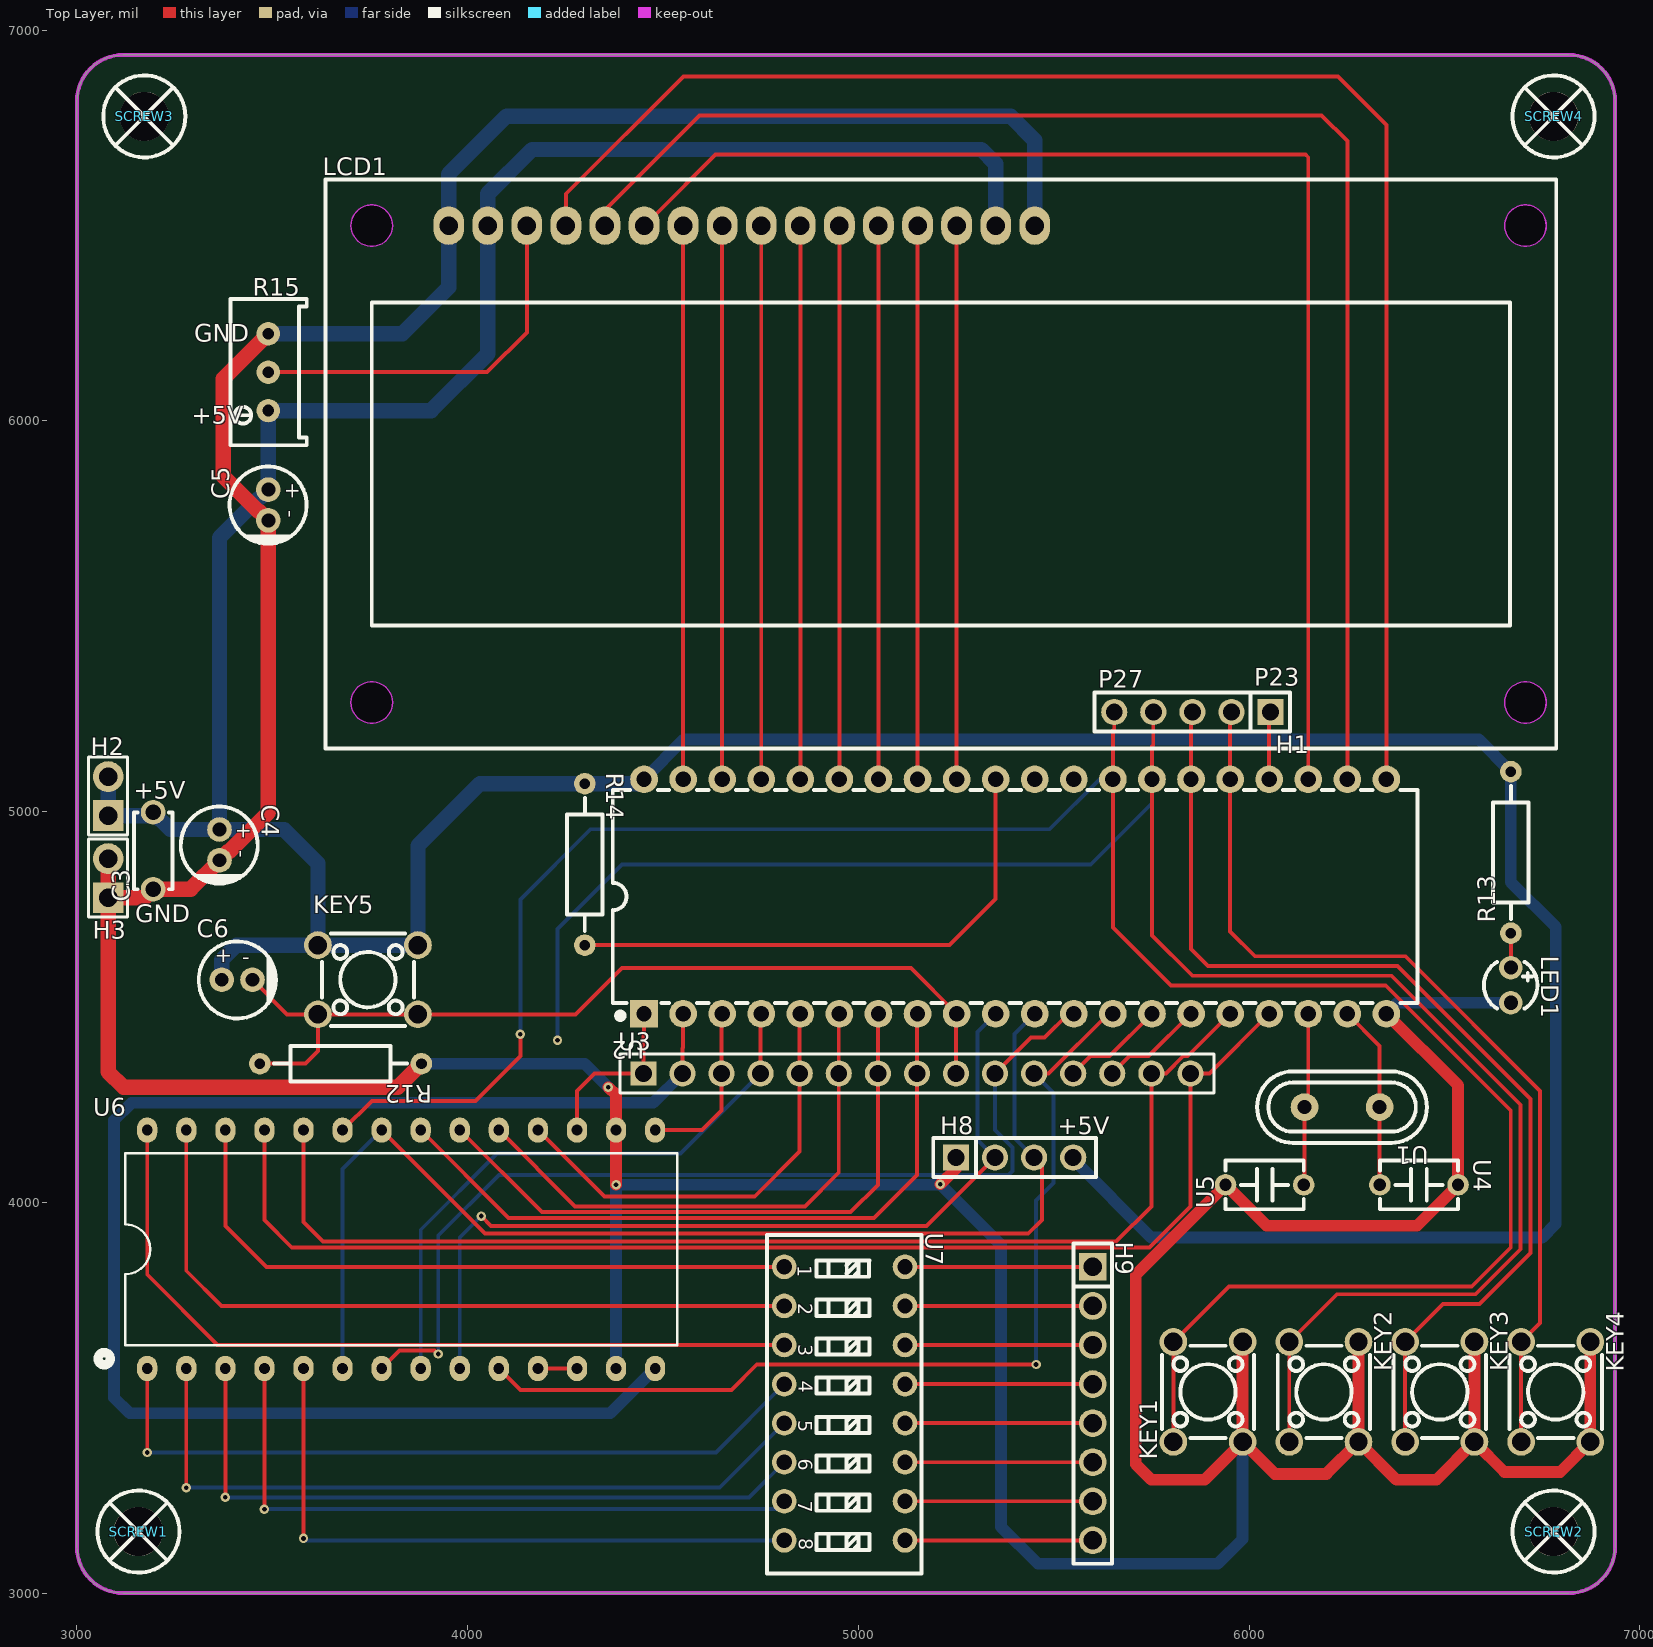
[diagram p0: Top Layer view]
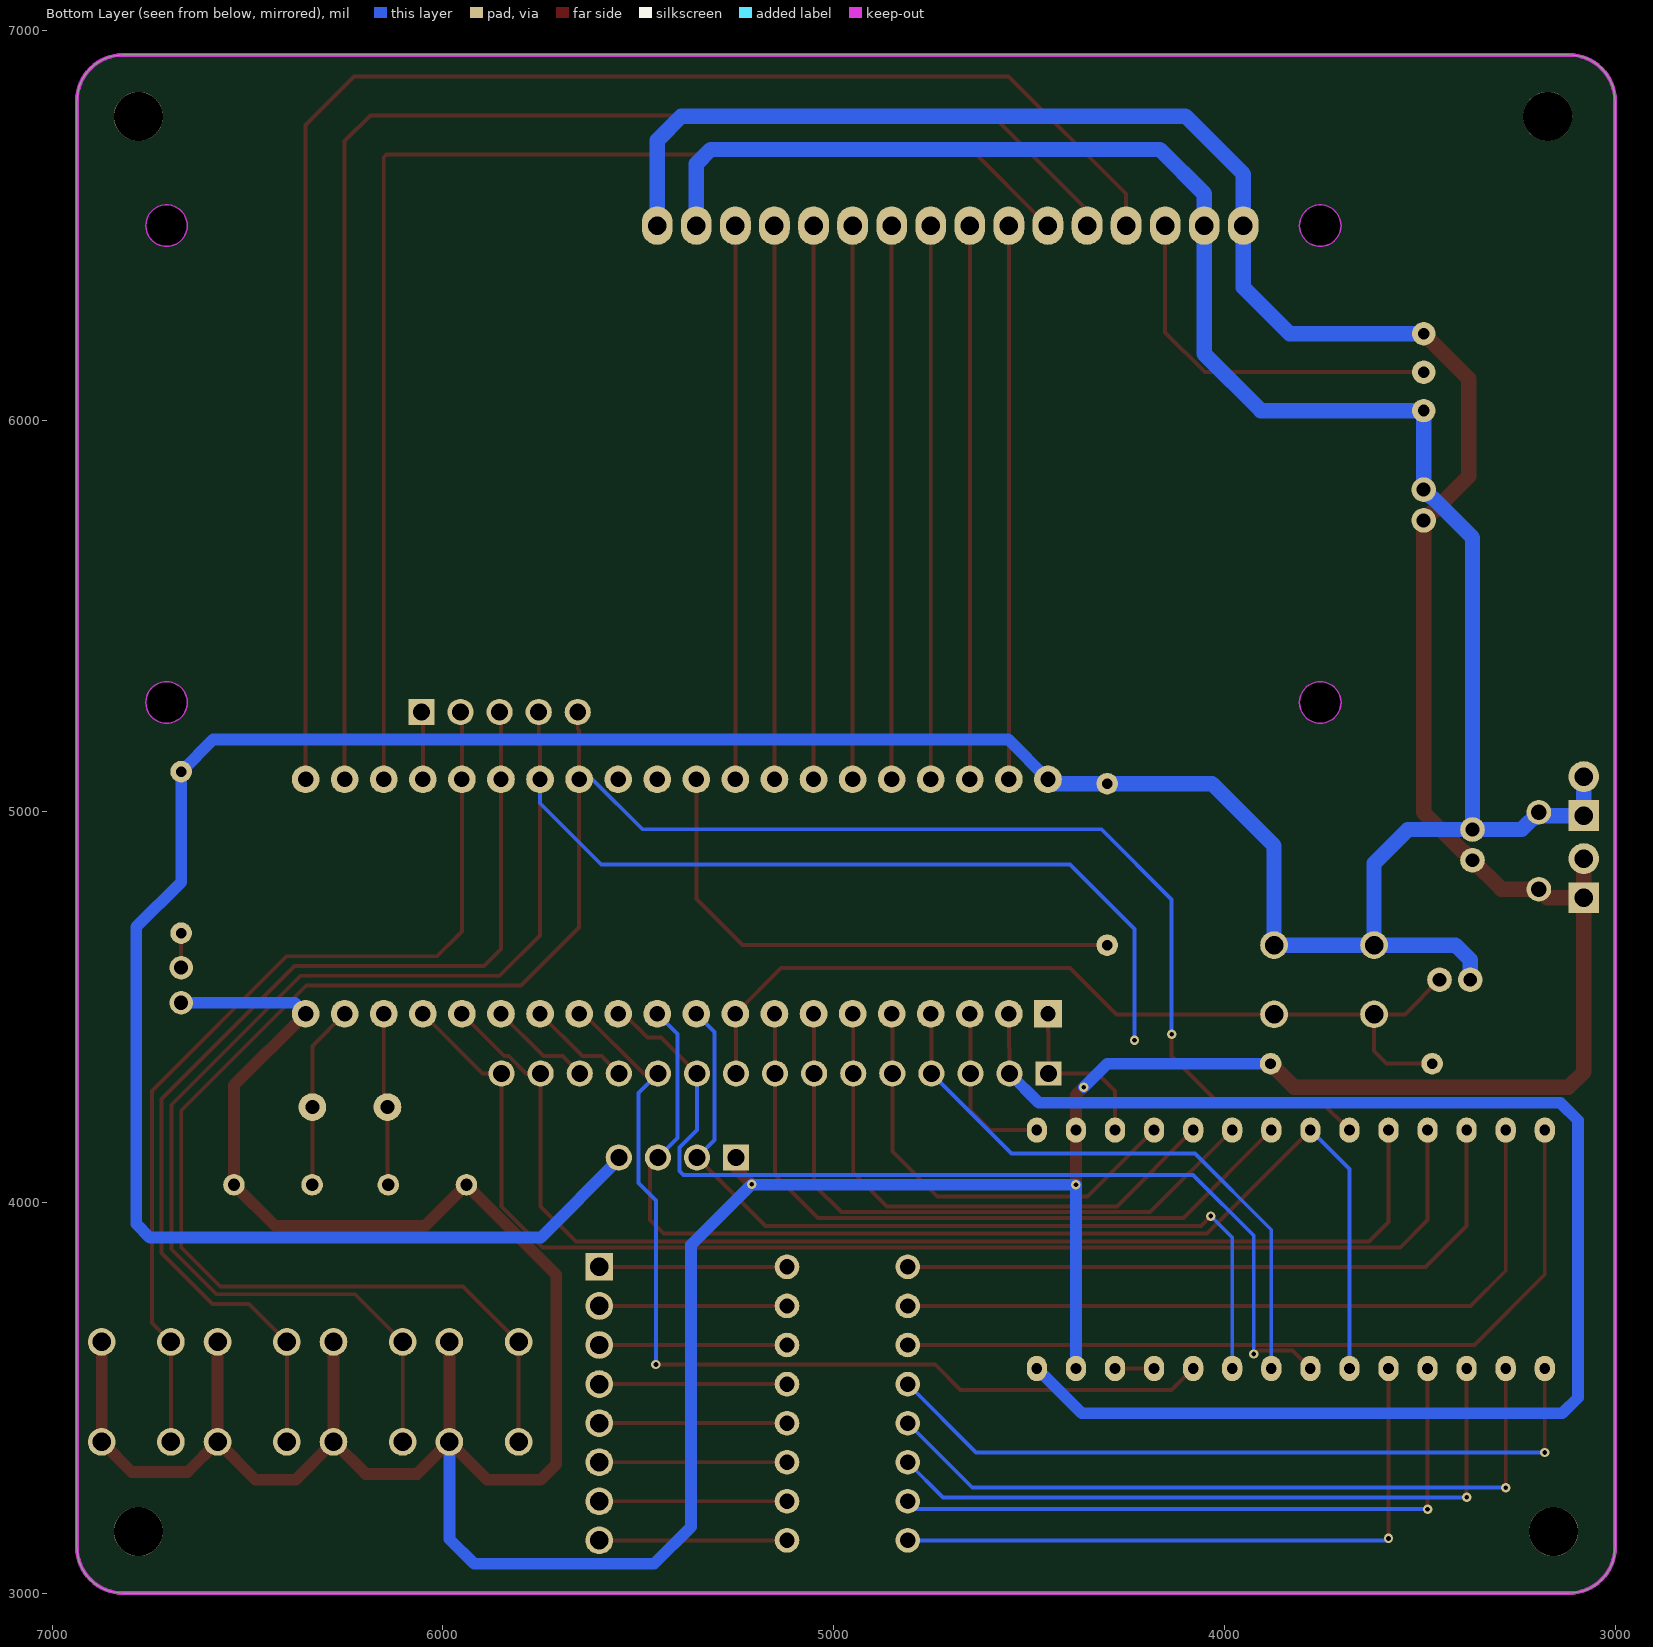
[diagram p1: Bottom Layer view, seen from below]
# Altium PCB MISC51962.pcbdoc
Units mil, origin at the board's own origin, x right, y up, seen from the top; angles counter-clockwise.
Board outline 3937.01 x 3937.01 mil, 2 copper layers (Top Layer, Bottom Layer), stack 62.206 mil thick; 31 components, 57 nets, 185 pads, 13 vias.

## Layer stack, top to bottom
Top Solder Mask Layer: solder mask 0.394, Dk 3.3
Top Layer: signal copper 1.379
Dielectric1: surface 59.449, FR4, Dk 4.5
Bottom Layer: signal copper 1.378
Bottom Solder Mask Layer: solder mask 0.394, Dk 3.3

## Board outline
3118.11,6937.01 ccw(c3118.11,6818.9) 3000,6818.9 3000,3118.11 ccw(c3118.11,3118.11) 3118.11,3000 6818.9,3000 ccw(c6818.9,3118.11) 6937.01,3118.11 6937.01,6818.9 ccw(c6818.9,6818.9) 6818.9,6937.01 3118.11,6937.01

## Design rules (kind name [scope] priority, off if disabled: settings)
BoardOutlineClearance copperThickness2oz_1 [All] p2 off: genericclearance=7.99 ignorepadtopadclearanceinfootprint=FALSE except(0: Arc-SplitContinuation Track-SplitContinuation SMDPad-SplitContinuation THPad-SplitContinuation Via-SplitContinuation Fill-SplitContinuation Region-SplitContinuation Poly-SplitContinuation Text-SplitContinuation Hole-SplitContinuation; 5.98: Arc-CutoutEdge Track-CutoutEdge SMDPad-CutoutEdge THPad-CutoutEdge Via-CutoutEdge Text-CutoutEdge; 6.9: Hole-OutlineEdge Hole-CutoutEdge; 10: Poly-OutlineEdge Poly-CutoutEdge; 11.81: Arc-OutlineEdge Track-OutlineEdge SMDPad-OutlineEdge THPad-OutlineEdge Via-OutlineEdge Fill-OutlineEdge Region-OutlineEdge Text-OutlineEdge Fill-CutoutEdge Region-CutoutEdge)
BoardOutlineClearance Plane_innerPlane_1 [All] p4 off: genericclearance=4.02 ignorepadtopadclearanceinfootprint=FALSE except(0: Arc-SplitContinuation Track-SplitContinuation SMDPad-SplitContinuation THPad-SplitContinuation Via-SplitContinuation Fill-SplitContinuation Region-SplitContinuation Poly-SplitContinuation Text-SplitContinuation Hole-SplitContinuation; 5.98: Arc-CutoutEdge Track-CutoutEdge SMDPad-CutoutEdge THPad-CutoutEdge Via-CutoutEdge Text-CutoutEdge; 6.9: Hole-OutlineEdge Hole-CutoutEdge; 10: Poly-OutlineEdge Poly-CutoutEdge; 11.81: Arc-OutlineEdge Track-OutlineEdge SMDPad-OutlineEdge THPad-OutlineEdge Via-OutlineEdge Fill-OutlineEdge Region-OutlineEdge Text-OutlineEdge Fill-CutoutEdge Region-CutoutEdge)
BoardOutlineClearance Copper_copperRegion_1 [All] p6 off: genericclearance=4.02 ignorepadtopadclearanceinfootprint=FALSE except(0: Arc-SplitContinuation Track-SplitContinuation SMDPad-SplitContinuation THPad-SplitContinuation Via-SplitContinuation Fill-SplitContinuation Region-SplitContinuation Poly-SplitContinuation Text-SplitContinuation Hole-SplitContinuation; 5.98: Arc-CutoutEdge Track-CutoutEdge SMDPad-CutoutEdge THPad-CutoutEdge Via-CutoutEdge Text-CutoutEdge; 6.9: Hole-OutlineEdge Hole-CutoutEdge; 10: Poly-OutlineEdge Poly-CutoutEdge; 11.81: Arc-OutlineEdge Track-OutlineEdge SMDPad-OutlineEdge THPad-OutlineEdge Via-OutlineEdge Fill-OutlineEdge Region-OutlineEdge Text-OutlineEdge Fill-CutoutEdge Region-CutoutEdge)
BoardOutlineClearance copperThickness1oz_1 [All] p8: genericclearance=4.02 ignorepadtopadclearanceinfootprint=FALSE except(0: Arc-SplitContinuation Track-SplitContinuation SMDPad-SplitContinuation THPad-SplitContinuation Via-SplitContinuation Fill-SplitContinuation Region-SplitContinuation Poly-SplitContinuation Text-SplitContinuation Hole-SplitContinuation; 5.98: Arc-CutoutEdge Track-CutoutEdge SMDPad-CutoutEdge THPad-CutoutEdge Via-CutoutEdge Text-CutoutEdge; 6.9: Hole-OutlineEdge Hole-CutoutEdge; 10: Poly-OutlineEdge Poly-CutoutEdge; 11.81: Arc-OutlineEdge Track-OutlineEdge SMDPad-OutlineEdge THPad-OutlineEdge Via-OutlineEdge Fill-OutlineEdge Region-OutlineEdge Text-OutlineEdge Fill-CutoutEdge Region-CutoutEdge)
Clearance copperThickness2oz [All] p1 off: gap=7.99 ignorepadtopadclearanceinfootprint=FALSE except(5.98: SMDPad-Track SMDPad-SMDPad THPad-Track SMDPad-THPad THPad-THPad Track-Via SMDPad-Via THPad-Via Via-Via Fill-SMDPad Region-SMDPad Fill-THPad Region-THPad Fill-Via Region-Via Fill-Fill Fill-Region Region-Region Arc-Track Arc-SMDPad Arc-THPad Arc-Via Fill-Arc Region-Arc Arc-Arc Text-Track SMDPad-Text Text-THPad Text-Via Fill-Text Region-Text Arc-Text Text-Text; 6.9: Hole-Track Hole-SMDPad Hole-THPad Hole-Via Fill-Hole Region-Hole Hole-Arc Hole-Text; 10: Poly-Track Poly-SMDPad Poly-THPad Poly-Via Poly-Fill Poly-Region Poly-Poly Poly-Arc Poly-Text Poly-Hole; 11.81: Fill-Track Region-Track)
Clearance Plane_innerPlane [All] p3 off: gap=4.02 ignorepadtopadclearanceinfootprint=FALSE except(5.98: SMDPad-Track SMDPad-SMDPad THPad-Track SMDPad-THPad THPad-THPad Track-Via SMDPad-Via THPad-Via Via-Via Fill-SMDPad Region-SMDPad Fill-THPad Region-THPad Fill-Via Region-Via Fill-Fill Fill-Region Region-Region Arc-Track Arc-SMDPad Arc-THPad Arc-Via Fill-Arc Region-Arc Arc-Arc Text-Track SMDPad-Text Text-THPad Text-Via Fill-Text Region-Text Arc-Text Text-Text; 6.9: Hole-Track Hole-SMDPad Hole-THPad Hole-Via Fill-Hole Region-Hole Hole-Arc Hole-Text; 10: Poly-Track Poly-SMDPad Poly-THPad Poly-Via Poly-Fill Poly-Region Poly-Poly Poly-Arc Poly-Text Poly-Hole; 11.81: Fill-Track Region-Track)
Clearance Copper_copperRegion [All] p5 off: gap=4.02 ignorepadtopadclearanceinfootprint=FALSE except(5.98: SMDPad-Track SMDPad-SMDPad THPad-Track SMDPad-THPad THPad-THPad Track-Via SMDPad-Via THPad-Via Via-Via Fill-SMDPad Region-SMDPad Fill-THPad Region-THPad Fill-Via Region-Via Fill-Fill Fill-Region Region-Region Arc-Track Arc-SMDPad Arc-THPad Arc-Via Fill-Arc Region-Arc Arc-Arc Text-Track SMDPad-Text Text-THPad Text-Via Fill-Text Region-Text Arc-Text Text-Text; 6.9: Hole-Track Hole-SMDPad Hole-THPad Hole-Via Fill-Hole Region-Hole Hole-Arc Hole-Text; 10: Poly-Track Poly-SMDPad Poly-THPad Poly-Via Poly-Fill Poly-Region Poly-Poly Poly-Arc Poly-Text Poly-Hole; 11.81: Fill-Track Region-Track)
Clearance copperThickness1oz [All] p7: gap=4.02 ignorepadtopadclearanceinfootprint=FALSE except(5.98: SMDPad-Track SMDPad-SMDPad THPad-Track SMDPad-THPad THPad-THPad Track-Via SMDPad-Via THPad-Via Via-Via Fill-SMDPad Region-SMDPad Fill-THPad Region-THPad Fill-Via Region-Via Fill-Fill Fill-Region Region-Region Arc-Track Arc-SMDPad Arc-THPad Arc-Via Fill-Arc Region-Arc Arc-Arc Text-Track SMDPad-Text Text-THPad Text-Via Fill-Text Region-Text Arc-Text Text-Text; 6.9: Hole-Track Hole-SMDPad Hole-THPad Hole-Via Fill-Hole Region-Hole Hole-Arc Hole-Text; 10: Poly-Track Poly-SMDPad Poly-THPad Poly-Via Poly-Fill Poly-Region Poly-Poly Poly-Arc Poly-Text Poly-Hole; 11.81: Fill-Track Region-Track)
DiffPairsRouting differentialPair [All] p1: maxlimit=6 minlimit=6 mostfreqgap=6 toplayer_minwidth=5 toplayer_prefwidth=10 toplayer_maxwidth=100 toplayer_mingap=6 toplayer_prefgap=6 toplayer_maxgap=6 bottomlayer_minwidth=5 bottomlayer_prefwidth=10 bottomlayer_maxwidth=100 bottomlayer_mingap=6 bottomlayer_prefgap=6 bottomlayer_maxgap=6 maxuncoupledlength=10
HoleToHoleClearance otherClearance [All] p1: gap=11.81 allowstackedmicrovias=TRUE
Length netLength [All] p1: minlimit=0 maxlimit=0
PasteMaskExpansion pasteMaskExpansion [All] p1: expansion=0
PlaneConnect innerPlane [All] p1: planeconnectstyle=Relief reliefexpansion=20 reliefentries=4 reliefconductorwidth=10 reliefairgap=10
PolygonConnect copperRegion [All] p1: connectstyle=Relief reliefconductorwidth=10 reliefentries=4 polygonreliefangle="90 Angle" airgapwidth=10 via.connectstyle=Relief via.reliefconductorwidth=10 via.reliefentries=4 via.polygonreliefangle="90 Angle" via.airgapwidth=10
RoutingVias viaSize [All] p1: holewidth=12.01 width=24.02 viastyle="Through Hole" minholewidth=11.81 minwidth=19.68 maxholewidth=248.03 maxwidth=393.7
SolderMaskExpansion solderMaskExpansion [IsVia] p1: expansion=-1000 istentingtop=TRUE
SolderMaskExpansion solderMaskExpansion [All] p2: expansion=2 istentingtop=FALSE
Width copperThickness2oz_2 [All] p1 off: maxlimit=100 minlimit=8 preferedwidth=10
Width copperThickness1oz_2 [All] p2: maxlimit=100 minlimit=5 preferedwidth=10

## Components (designator, comment, footprint, x,y, rotation, side; value= is the part's Value field where it differs from the comment)
C3 "100nF" CAP-TH_L5.0-W2.5-P5.00-D1.0 3195,4900 r90 top
C4 "10uF" CAP-TH_BD5.0-P2.00-D0.5-FD-A 3365,4915 r270 top
C5 "10uF" CAP-TH_BD5.0-P2.00-D0.5-FD-A 3490,5785 r270 top
C6 "10uF" CAP-TH_BD5.0-P2.00-D0.5-FD-A 3410,4570 r0 top
H1 "PZ254V-11-05P" HDR-TH_5P-P2.54-V-M 5855,5255 r180 top
H2 "PZ254V-11-02P" HDR-TH_2P-P2.54-V-M 3080,5040 r90 top
H3 "PZ254V-11-02P" HDR-TH_2P-P2.54-V-M 3080,4830 r90 top
H8 "" HDR-TH_4P-P2.54-V-F 5400,4115 r0 top
H9 "" HDR-TH_8P-P2.54-V-F-1 5600,3485 r270 top
KEY1 "" SW-TH_4P-L6.0-W6.0-P4.50-LS6.5 5895,3515 r270 top
KEY2 "" SW-TH_4P-L6.0-W6.0-P4.50-LS6.5 6191.67,3515 r270 top
KEY3 "" SW-TH_4P-L6.0-W6.0-P4.50-LS6.5 6488.33,3515 r270 top
KEY4 "" SW-TH_4P-L6.0-W6.0-P4.50-LS6.5 6785,3515 r270 top
KEY5 "" SW-TH_4P-L6.0-W6.0-P4.50-LS6.5 3745,4570 r180 top
LCD1 "LCM1602K-NSW-BBW" MODULE-TH_LCM1602K 4701.61,6500 r0 top
LED1 "3A2RUD" LED-TH_BD3.5-P2.28_3A2RUC 6670.18,4555.82 r270 top
R12 "10kΩ" RES-TH_BD2.3-L6.5-P10.50-D0.5 3675,4355 r180 top
R13 "10kΩ" RES-TH_BD2.3-L6.5-P10.50-D0.5 6670.18,4895.82 r90 top
R14 "10kΩ" RES-TH_BD2.3-L6.5-P10.50-D0.5 4300,4865 r270 top
R15 "10kΩ" RES-ADJ-TH_3P-L10.0-W10.0-P2.50-L 3490,6125 r90 top
SCREW1 "" M3螺丝 3157.48,3157.48 r0 top
SCREW2 "" M3螺丝 6779.53,3157.48 r0 top
SCREW3 "" M3螺丝 3172.48,6779.53 r0 top
SCREW4 "" M3螺丝 6779.53,6779.53 r0 top
U1 "12MHz" HC-49S_L11.0-W4.7-P4.88 6238.18,4243.91 r180 top
U2 "STC89C516RD+40I-PDIP40" DIP-40_L52.3-W13.9-P2.54-LS15.2-BL 5401.61,4782.88 r0 top
U3 "ZX-PM2.54-1-15PY" HDR-TH_15P-P2.54-V-F 5150,4330 r0 top
U4 "33pF" CAP-TH_L5.0-W2.5-P5.08-D0.7 6435,4045 r180 top
U5 "33pF" CAP-TH_L5.0-W2.5-P5.08-D0.7 6040,4045 r0 top
U6 "ADC0809-N" PDIP-28_L36.0-W13.0-P2.54-LS15.5-BL 3830,3880 r0 top
U7 "2.54插件8位拨码开关" SW-TH_16P-L21.9-W9.9-P2.54-LS7.8 4965,3485 r270 top

## Footprints (in the part's own frame and the unit in brackets; to place one, negate y for a bottom-side part, rotate by r counter-clockwise, add the part's x,y. Pads: shape width x height; smd on the part's side, far side on the other; paste and mask are expansions set on the pad)
CAP-TH_BD5.0-P2.00-D0.5-FD-A [mm]
  round 1.6 hole 0.9 paste+0 mask+0.05: 1(-1,0) 2(1,0)
  silkscreen extent -2.49,-2.52 2.6,2.49
CAP-TH_L5.0-W2.5-P5.00-D1.0 [mm]
  round 1.6 hole 1: 1(-2.5,0) 2(2.5,0)
  silkscreen extent -2.5,-1.27 2.5,1.25
CAP-TH_L5.0-W2.5-P5.08-D0.7 [mm]
  round 1.4 hole 0.8: 1(-2.54,0) 2(2.54,0)
  silkscreen extent -2.54,-1.59 2.54,1.59
DIP-40_L52.3-W13.9-P2.54-LS15.2-BL [mm]
  rect 1.8x1.8 hole 1: 1(-24.13,-7.62)
  round 1.8 hole 1: 2(-21.59,-7.62) 3(-19.05,-7.62) 4(-16.51,-7.62) 5(-13.97,-7.62) 6(-11.43,-7.62) 7(-8.89,-7.62) 8(-6.35,-7.62) 9(-3.81,-7.62) 10(-1.27,-7.62) 11(1.27,-7.62) 12(3.81,-7.62) 13(6.35,-7.62) 14(8.89,-7.62) 15(11.43,-7.62) 16(13.97,-7.62) 17(16.51,-7.62) 18(19.05,-7.62) 19(21.59,-7.62) 20(24.13,-7.62) 21(24.13,7.62) 22(21.59,7.62) 23(19.05,7.62) 24(16.51,7.62) 25(13.97,7.62) 26(11.43,7.62) 27(8.89,7.62) 28(6.35,7.62) 29(3.81,7.62) 30(1.27,7.62) 31(-1.27,7.62) 32(-3.81,7.62) 33(-6.35,7.62) 34(-8.89,7.62) 35(-11.43,7.62) 36(-13.97,7.62) 37(-16.51,7.62) 38(-19.05,7.62) 39(-21.59,7.62) 40(-24.13,7.62)
  silkscreen extent -26.16,-7.95 26.16,6.93
HC-49S_L11.0-W4.7-P4.88 [mm]
  round 1.8 hole 0.9: 1(-2.44,0) 2(2.44,0)
  silkscreen extent -5.52,-2.32 5.52,2.33
HDR-TH_2P-P2.54-V-M [mm]
  rect 2x2 hole 1.2: 1(-1.27,0)
  round 2 hole 1.2: 2(1.27,0)
  silkscreen extent -2.54,-1.27 2.54,1.27
HDR-TH_4P-P2.54-V-F [mm]
  rect 1.7x1.7 hole 1.1: 1(-3.81,0)
  round 1.7 hole 1.1: 2(-1.27,0) 3(1.27,0) 4(3.81,0)
  silkscreen extent -5.29,-1.27 5.29,1.27
HDR-TH_5P-P2.54-V-M [mm]
  rect 1.7x1.7 hole 1.1: 1(-5.08,0)
  round 1.7 hole 1.1: 2(-2.54,0) 3(0,0) 4(2.54,0) 5(5.08,0)
  silkscreen extent -6.35,-1.27 6.35,1.27
HDR-TH_8P-P2.54-V-F-1 [mm]
  rect 1.8x1.8 hole 1.2: 1(-8.89,0)
  round 1.8 hole 1.2: 2(-6.35,0) 3(-3.81,0) 4(-1.27,0) 5(1.27,0) 6(3.81,0) 7(6.35,0) 8(8.89,0)
  silkscreen extent -10.41,-1.25 10.41,1.25
HDR-TH_15P-P2.54-V-F [mm]
  rect 1.7x1.575 hole 1.1: 1(-17.78,0)
  round 1.7 hole 1.1: 2(-15.24,0) 3(-12.7,0) 4(-10.16,0) 5(-7.62,0) 6(-5.08,0) 7(-2.54,0) 8(0,0) 9(2.54,0) 10(5.08,0) 11(7.62,0) 12(10.16,0) 13(12.7,0) 14(15.24,0) 15(17.78,0)
  silkscreen extent -19.3,-1.27 19.3,1.27
LED-TH_BD3.5-P2.28_3A2RUC [mil]
  round 60 hole 36: 1(44.88,0) 2(-44.88,0)
  silkscreen extent -60,-69 60,68
M3螺丝 [mil]
  round 126 hole 126 paste+0 mask+4: 1(0,0)
  silkscreen extent -105,-105 105,105
MODULE-TH_LCM1602K [mm]
  oval 2x2.5 hole 1.2: 1(-19.05,0) 2(-16.51,0) 3(-13.97,0) 4(-11.43,0) 5(-8.89,0) 6(-6.35,0) 7(-3.81,0) 8(-1.27,0) 9(1.27,0) 10(3.81,0) 11(6.35,0) 12(8.89,0) 13(11.43,0) 14(13.97,0) 15(16.51,0) 16(19.05,0)
  Board Outline Layer circle w0.003: c-24.051,0 r1.35
  Board Outline Layer circle w0.003: c50.95,0 r1.35
  Board Outline Layer circle w0.003: c50.95,-31.001 r1.35
  Board Outline Layer circle w0.003: c-24.051,-31.001 r1.35
  Board Outline Layer region: -22.701,0 -22.835,-0.586 -23.21,-1.055 -23.751,-1.316 -24.352,-1.316 -24.893,-1.055 -25.268,-0.586 -25.401,0 -25.401,0 -25.268,0.586 -24.893,1.055 -24.352,1.316 -23.751,1.316 -23.21,1.055 -22.835,0.586 -22.701,0
  Board Outline Layer region: -22.701,0 -22.711,-0.163 -22.74,-0.323 -22.789,-0.479 -22.856,-0.627 -22.94,-0.767 -23.041,-0.895 -23.156,-1.01 -23.284,-1.111 -23.424,-1.195 -23.573,-1.262 -23.728,-1.311 -23.889,-1.34 -24.051,-1.35 -24.214,-1.34 -24.374,-1.311 -24.53,-1.262 -24.679,-1.195 -24.818,-1.111 -24.946,-1.01 -25.062,-0.895 -25.162,-0.767 -25.247,-0.627 -25.314,-0.479 -25.362,-0.323 -25.391,-0.163 -25.401,0 -25.391,0.163 -25.362,0.323 -25.314,0.479 -25.247,0.627 -25.162,0.767 -25.062,0.895 -24.946,1.01 -24.818,1.111 -24.679,1.195 -24.53,1.262 -24.374,1.311 -24.214,1.34 -24.051,1.35 -23.889,1.34 -23.728,1.311 -23.573,1.262 -23.424,1.195 -23.284,1.111 -23.156,1.01 -23.041,0.895 -22.94,0.767 -22.856,0.627 -22.789,0.479 -22.74,0.323 -22.711,0.163
  Board Outline Layer region: 52.3,0 52.166,-0.586 51.792,-1.055 51.25,-1.316 50.649,-1.316 50.108,-1.055 49.734,-0.586 49.6,0 49.6,0 49.734,0.586 50.108,1.055 50.649,1.316 51.25,1.316 51.792,1.055 52.166,0.586 52.3,0
  Board Outline Layer region: 52.3,0 52.29,-0.163 52.261,-0.323 52.212,-0.479 52.145,-0.627 52.061,-0.767 51.96,-0.895 51.845,-1.01 51.717,-1.111 51.577,-1.195 51.429,-1.262 51.273,-1.311 51.113,-1.34 50.95,-1.35 50.787,-1.34 50.627,-1.311 50.471,-1.262 50.322,-1.195 50.183,-1.111 50.055,-1.01 49.939,-0.895 49.839,-0.767 49.754,-0.627 49.688,-0.479 49.639,-0.323 49.61,-0.163 49.6,0 49.61,0.163 49.639,0.323 49.688,0.479 49.754,0.627 49.839,0.767 49.939,0.895 50.055,1.01 50.183,1.111 50.322,1.195 50.471,1.262 50.627,1.311 50.787,1.34 50.95,1.35 51.113,1.34 51.273,1.311 51.429,1.262 51.577,1.195 51.717,1.111 51.845,1.01 51.96,0.895 52.061,0.767 52.145,0.627 52.212,0.479 52.261,0.323 52.29,0.163
  Board Outline Layer region: 52.3,-31.001 52.166,-31.586 51.792,-32.056 51.25,-32.317 50.649,-32.317 50.108,-32.056 49.734,-31.586 49.6,-31.001 49.6,-31.001 49.734,-30.415 50.108,-29.945 50.649,-29.685 51.25,-29.685 51.792,-29.945 52.166,-30.415 52.3,-31.001
  Board Outline Layer region: 52.3,-31.001 52.29,-31.163 52.261,-31.324 52.212,-31.479 52.145,-31.628 52.061,-31.768 51.96,-31.896 51.845,-32.011 51.717,-32.112 51.577,-32.196 51.429,-32.263 51.273,-32.311 51.113,-32.341 50.95,-32.351 50.787,-32.341 50.627,-32.311 50.471,-32.263 50.322,-32.196 50.183,-32.112 50.055,-32.011 49.939,-31.896 49.839,-31.768 49.754,-31.628 49.688,-31.479 49.639,-31.324 49.61,-31.163 49.6,-31.001 49.61,-30.838 49.639,-30.678 49.688,-30.522 49.754,-30.373 49.839,-30.234 49.939,-30.105 50.055,-29.99 50.183,-29.89 50.322,-29.805 50.471,-29.738 50.627,-29.69 50.787,-29.661 50.95,-29.651 51.113,-29.661 51.273,-29.69 51.429,-29.738 51.577,-29.805 51.717,-29.89 51.845,-29.99 51.96,-30.105 52.061,-30.234 52.145,-30.373 52.212,-30.522 52.261,-30.678 52.29,-30.838
  Board Outline Layer region: -22.701,-31.001 -22.835,-31.586 -23.21,-32.056 -23.751,-32.317 -24.352,-32.317 -24.893,-32.056 -25.268,-31.586 -25.401,-31.001 -25.401,-31.001 -25.268,-30.415 -24.893,-29.945 -24.352,-29.685 -23.751,-29.685 -23.21,-29.945 -22.835,-30.415 -22.701,-31.001
  Board Outline Layer region: -22.701,-31.001 -22.711,-31.163 -22.74,-31.324 -22.789,-31.479 -22.856,-31.628 -22.94,-31.768 -23.041,-31.896 -23.156,-32.011 -23.284,-32.112 -23.424,-32.196 -23.573,-32.263 -23.728,-32.311 -23.889,-32.341 -24.051,-32.351 -24.214,-32.341 -24.374,-32.311 -24.53,-32.263 -24.679,-32.196 -24.818,-32.112 -24.946,-32.011 -25.062,-31.896 -25.162,-31.768 -25.247,-31.628 -25.314,-31.479 -25.362,-31.324 -25.391,-31.163 -25.401,-31.001 -25.391,-30.838 -25.362,-30.678 -25.314,-30.522 -25.247,-30.373 -25.162,-30.234 -25.062,-30.105 -24.946,-29.99 -24.818,-29.89 -24.679,-29.805 -24.53,-29.738 -24.374,-29.69 -24.214,-29.661 -24.051,-29.651 -23.889,-29.661 -23.728,-29.69 -23.573,-29.738 -23.424,-29.805 -23.284,-29.89 -23.156,-29.99 -23.041,-30.105 -22.94,-30.234 -22.856,-30.373 -22.789,-30.522 -22.74,-30.678 -22.711,-30.838
  Multi-Layer board cut-out: -22.701,0 -22.835,-0.586 -23.21,-1.055 -23.751,-1.316 -24.352,-1.316 -24.893,-1.055 -25.268,-0.586 -25.401,0 -25.401,0 -25.268,0.586 -24.893,1.055 -24.352,1.316 -23.751,1.316 -23.21,1.055 -22.835,0.586 -22.701,0
  Multi-Layer board cut-out: 52.3,0 52.166,-0.586 51.792,-1.055 51.25,-1.316 50.649,-1.316 50.108,-1.055 49.734,-0.586 49.6,0 49.6,0 49.734,0.586 50.108,1.055 50.649,1.316 51.25,1.316 51.792,1.055 52.166,0.586 52.3,0
  Multi-Layer board cut-out: 52.3,-31.001 52.166,-31.586 51.792,-32.056 51.25,-32.317 50.649,-32.317 50.108,-32.056 49.734,-31.586 49.6,-31.001 49.6,-31.001 49.734,-30.415 50.108,-29.945 50.649,-29.685 51.25,-29.685 51.792,-29.945 52.166,-30.415 52.3,-31.001
  Multi-Layer board cut-out: -22.701,-31.001 -22.835,-31.586 -23.21,-32.056 -23.751,-32.317 -24.352,-32.317 -24.893,-32.056 -25.268,-31.586 -25.401,-31.001 -25.401,-31.001 -25.268,-30.415 -24.893,-29.945 -24.352,-29.685 -23.751,-29.685 -23.21,-29.945 -22.835,-30.415 -22.701,-31.001
  silkscreen extent -27.05,-34 52.95,3
PDIP-28_L36.0-W13.0-P2.54-LS15.5-BL [mil]
  oval 51.73x64.67 hole 27.56: 1(-650,-305.02) 2(-550,-305.02) 3(-450,-305.02) 4(-350,-305.02) 5(-250,-305.02) 6(-150,-305.02) 7(-50,-305.02) 8(50,-305.02) 9(150,-305.02) 10(250,-305.02) 11(350,-305.02) 12(450,-305.02) 13(550,-305.02) 14(650,-305.02) 15(650,305.02) 16(550,305.02) 17(450,305.02) 18(350,305.02) 19(250,305.02) 20(150,305.02) 21(50,305.02) 22(-50,305.02) 23(-150,305.02) 24(-250,305.02) 25(-350,305.02) 26(-450,305.02) 27(-550,305.02) 28(-650,305.02)
  silkscreen extent -776,-296 706,246
RES-ADJ-TH_3P-L10.0-W10.0-P2.50-L [mil]
  round 60 hole 30: 1(-98.43,0) 2(0,0) 3(98.43,0)
  silkscreen extent -187,-98 187,96
RES-TH_BD2.3-L6.5-P10.50-D0.5 [mm]
  round 1.4 hole 0.7: 1(-5.25,0) 2(5.25,0)
  silkscreen extent -4.32,-1.15 4.32,1.15
SW-TH_4P-L6.0-W6.0-P4.50-LS6.5 [mm]
  round 1.8 hole 1.2: 1(-3.25,2.25) 2(3.25,2.25) 3(-3.25,-2.25) 4(3.25,-2.25)
  silkscreen extent -3,-3 3,3
SW-TH_16P-L21.9-W9.9-P2.54-LS7.8 [mm]
  round 1.6 hole 1 paste+0 mask+0.05: 1(-8.89,-3.925) 2(-6.35,-3.925) 3(-3.81,-3.925) 4(-1.27,-3.925) 5(1.27,-3.925) 6(3.81,-3.925) 7(6.35,-3.925) 8(8.89,-3.925) 9(8.89,3.925) 10(6.35,3.925) 11(3.81,3.925) 12(1.27,3.925) 13(-1.27,3.925) 14(-3.81,3.925) 15(-6.35,3.925) 16(-8.89,3.925)
  silkscreen extent -10.97,-5.05 11.05,5.01

## Via types
v1: diameter 24.02, hole 12, Top Layer to Bottom Layer, 13 vias

## Nets (pads, with @x,y where several pads share a name; then routed paths per layer and width w, separated by ;. In a path a pad name is that pad's centre, name@x,y a point inside that pad or via, vN(x,y) a via of type N, cw(c..) or ccw(c..) an arc to the next point about the centre after c; other vN are vias at no path point)
$1N854: LED1.2 R13.1 | length 88.4
  Top Layer w10: LED1.2 R13.1
$1N1184: R14.2 U2.31 | length 1406.9
  Top Layer w10: R14.2 5233.31,4658.31 5351.61,4776.61 U2.31
$1N2217: LCD1.3 R15.2 | length 977.1
  Top Layer w10: R15.2 4050.01,6125.01 4151.61,6226.61 LCD1.3
$1N10346: U6.1 U7.4 | length 1917.9
  Top Layer w10: v1(3180,3360) U6.1
  Bottom Layer w10: v1(3180,3360) 4635.47,3360 U7.4
$1N10348: U6.2 U7.5 | length 1903.8
  Top Layer w10: v1(3280,3270) U6.2
  Bottom Layer w10: v1(3280,3270) 4645.47,3270 U7.5
$1N10350: U6.3 U7.6 | length 1797.7
  Top Layer w10: v1(3380,3245) U6.3
  Bottom Layer w10: v1(3380,3245) 4720.47,3245 U7.6
$1N10352: U6.4 U7.7 | length 1698.7
  Top Layer w10: v1(3480,3215) U6.4
  Bottom Layer w10: v1(3480,3215) 4790.47,3215 U7.7
$1N10354: U6.5 U7.8 | length 1667.5
  Top Layer w10: v1(3580,3140) U6.5
  Bottom Layer w10: v1(3580,3140) 3585,3135 U7.8
$1N10356: U6.26 U7.1 | length 1719
  Top Layer w10: U6.26 3380,3940 3485,3835 U7.1
$1N10358: U6.27 U7.2 | length 1927.8
  Top Layer w10: U6.27 3280,3825 3370,3735 U7.2
$1N10360: U6.28 U7.3 | length 2075
  Top Layer w10: U6.28 3180,3815 3360,3635 U7.3
$1N10829: H9.8 U7.9 | length 480.5
  Top Layer w10: U7.9 H9.8
$1N10831: H9.7 U7.10 | length 480.5
  Top Layer w10: U7.10 H9.7
$1N10833: H9.6 U7.11 | length 480.5
  Top Layer w10: U7.11 H9.6
$1N10835: H9.5 U7.12 | length 480.5
  Top Layer w10: U7.12 H9.5
$1N10837: H9.4 U7.13 | length 480.5
  Top Layer w10: U7.13 H9.4
$1N10839: H9.3 U7.14 | length 480.5
  Top Layer w10: U7.14 H9.3
$1N10841: H9.2 U7.15 | length 480.5
  Top Layer w10: U7.15 H9.2
$1N10843: H9.1 U7.16 | length 480.5
  Top Layer w10: U7.16 H9.1
+5V: C3.2 C4.1 C5.1 C6.1 H2.1 H2.2 H8.4 KEY5.3 KEY5.4 LCD1.2 LCD1.15 R13.2 R14.1 R15.1 U2.40 | length 10890.9
  Bottom Layer w30: U2.40 4553.73,5185 6587.69,5185 R13.2 6670.18,4819.82 6785,4705 6785,3945 6750,3910 5750,3910 5550,4110 H8.4
  Bottom Layer w39.37: H2.2 H2.1 3186.57,4990 C3.2 3239.05,4954.37 C4.1 ; C6.1 3370.63,4620.63 3408.58,4658.58 KEY5.4 ; U2.40 4440.42,5071.69 R14.1 4031.69,5071.69 3872.95,4912.95 KEY5.3 KEY5.4 ; LCD1.15 5351.61,6658.39 5315,6695 4165,6695 4051.61,6581.61 LCD1.2 4051.61,6171.61 3906.57,6026.57 R15.1 C5.1 3468.42,5802.8 3466.32,5802.8 3365,5701.47 C4.1 ; C4.1 3530.63,4954.37 3617.05,4867.95 KEY5.4
GND: C3.1 C4.2 C5.2 H3.1 H3.2 H8.1 KEY1.1 KEY1.2 KEY2.1 KEY2.2 KEY3.1 KEY3.2 KEY4.1 KEY4.2 LCD1.1 LCD1.16 LED1.1 R12.1 R15.3 U2.20 U4.1 U5.1 U6.13 U6.16 | length 14629.4
  Top Layer w30: v1(4360,4295) 4380,4275 U6.16 v1(4380,4045) ; v1(5210,4046.54) 5250,4086.54 H8.1 ; KEY1.1 KEY1.2 ; KEY2.1 KEY2.2 ; U2.20 6535,4299.48 U4.1 6430,3940 6045,3940 U5.1 5710,3815 5710,3330 5750,3290 5886.53,3290 KEY1.2 ; KEY3.1 KEY3.2 ; KEY4.1 KEY4.2 6796.53,3310 6653.96,3310 KEY3.2 ; KEY1.2 6065.63,3305 6198.2,3305 KEY2.2 ; KEY2.2 6377.3,3290 6479.86,3290 KEY3.2
  Top Layer w39.37: H3.2 H3.1 ; R15.3 3375,6108.43 3375,5858.52 3466.32,5767.2 3468.42,5767.2 C5.2 3490,4998.53 3388.67,4897.2 3386.57,4897.2 C4.2 3290.94,4801.57 C3.1 3173.43,4780 H3.1 ; R12.1 3821.69,4295 3119.37,4295 3080,4334.37 H3.1
  Bottom Layer w30: R12.1 4300,4355 v1(4360,4295) ; U6.13 v1(4380,4045) 5208.46,4045 v1(5210,4046.54) 5365,3891.54 5365,3170 5460,3075 5920,3075 5983.58,3138.58 KEY1.2 ; U2.20 6379.67,4510.94 LED1.1
  Bottom Layer w39.37: R15.3 3833.43,6223.43 3951.61,6341.61 LCD1.1 3951.61,6631.61 4100,6780 5390,6780 5451.61,6718.39 LCD1.16
P00: LCD1.7 U2.39 | length 1417.1
  Top Layer w10: U2.39 LCD1.7
P01: LCD1.8 U2.38 | length 1417.1
  Top Layer w10: U2.38 LCD1.8
P02: LCD1.9 U2.37 | length 1417.1
  Top Layer w10: U2.37 LCD1.9
P03: LCD1.10 U2.36 | length 1417.1
  Top Layer w10: U2.36 LCD1.10
P04: LCD1.11 U2.35 | length 1417.1
  Top Layer w10: U2.35 LCD1.11
P05: LCD1.12 U2.34 | length 1417.1
  Top Layer w10: U2.34 LCD1.12
P06: LCD1.13 U2.33 | length 1417.1
  Top Layer w10: U2.33 LCD1.13
P07: LCD1.14 U2.32 | length 1417.1
  Top Layer w10: U2.32 LCD1.14
P10: U2.1 U3.1 U6.17 | length 442.2
  Top Layer w10: U6.17 4280,4285 4325,4330 U3.1 4450,4435.83 4451.61,4437.44 U2.1
P11: U2.2 U3.2 U6.14 | length 3817.4
  Top Layer w10: U3.2 4550,4394.41 4551.61,4396.02 U2.2
  Bottom Layer w30: U6.14 4365.02,3460 3135,3460 3095,3500 3095,4210 3140,4255 4475,4255 U3.2
P12: U2.3 U3.3 U6.15 | length 439.2
  Top Layer w10: U6.15 4600.02,4185.02 4650,4235 U3.3 4650,4481.27 U2.3
P13: U2.4 U3.4 U6.8 | length 1544.2
  Top Layer w10: U3.4 4750,4481.27 U2.4
  Bottom Layer w10: U6.8 3880,3930 4075,4125 4545,4125 U3.4
P14: U2.5 U3.5 U6.18 | length 1141.6
  Top Layer w10: U6.18 4350.02,4015 4735,4015 4850,4130 U3.5 4850,4481.27 U2.5
P15: U2.6 U3.6 U6.19 | length 1393.6
  Top Layer w10: U6.19 4275.02,3990 4863.43,3990 4950,4076.57 U3.6 4950,4481.27 U2.6
P16: U2.7 U3.7 U6.20 | length 1624.5
  Top Layer w10: U6.20 4190.02,3975 4980,3975 5050,4045 U3.7 5050,4481.27 U2.7
P17: U2.8 U3.8 U6.21 | length 1822.3
  Top Layer w10: U6.21 4105.02,3960 5040,3960 5150,4070 U3.8 5150,4481.27 U2.8
P20: LCD1.4 U2.21 | length 4032.5
  Top Layer w10: LCD1.4 4251.61,6581.61 4552.07,6882.07 6227.38,6882.07 6351.61,6757.84 U2.21
P21: LCD1.5 U2.22 | length 3701.1
  Top Layer w10: LCD1.5 4351.61,6540.19 4593.49,6782.07 6185.96,6782.07 6251.61,6716.42 U2.22
P22: LCD1.6 U2.23 | length 3335.9
  Top Layer w10: LCD1.6@4476.42,6523.58 4634.91,6682.07 6144.54,6682.07 6151.61,6675 U2.23
P23: H1.1 U2.24 | length 173.5
  Top Layer w10: U2.24 6051.61,5251.61 H1.1
P24: H1.2 KEY4.3 KEY4.4 U2.25 | length 2443.6
  Top Layer w10: H1.2 5951.61,5251.61 U2.25 5951.61,4693.39 6015,4630 6400,4630 6745,4285 6745,3691.53 KEY4.3 KEY4.4
P25: H1.3 KEY3.3 KEY3.4 U2.26 | length 2700.4
  Top Layer w10: H1.3 5851.61,5251.61 U2.26 5851.61,4648.39 5895,4605 6380,4605 6720,4265 6720,3870 6590,3740 6496.8,3740 KEY3.3 KEY3.4
P26: H1.4 KEY2.3 KEY2.4 U2.27 | length 5013
  Top Layer w10: H1.4 5755,5170.11 5751.61,5166.72 U2.27 5751.61,4683.39 5855,4580 6365,4580 6695,4250 6695,3880 6580,3765 6225.14,3765 KEY2.3 KEY2.4
  Bottom Layer w10: v1(4230,4415) 4230,4700 4395,4865 5595,4865 5751.61,5021.61 U2.27
P27: H1.5 KEY1.3 KEY1.4 U2.28 U6.23 | length 5913
  Top Layer w10: U6.23 3754.98,4260 4020,4260 4135,4375 v1(4135,4430) ; H1.5 5655,5211.54 5651.61,5208.14 U2.28 5651.61,4703.39 5800,4555 6350,4555 6670,4235 6670,3885 6570,3785 5948.47,3785 KEY1.3 KEY1.4
  Bottom Layer w10: v1(4135,4430) 4135,4775 4315,4955 5489.38,4955 5617.25,5082.88 U2.28
P30: H8.2 U2.10 U6.9 | length 2216.5
  Top Layer w10: v1(4035,3965) 4060,3940 5175,3940 H8.2
  Bottom Layer w10: U6.9 3980,3910 v1(4035,3965) ; H8.2 5305,4160 5305,4436.27 U2.10
P31: H8.3 U2.11 U6.6 U6.22 | length 3044
  Top Layer w10: U6.22 4045.02,3920 5435,3920 5470,3955 5470,4095 H8.3
  Bottom Layer w10: U6.6 3680,4085.02 U6.22 ; H8.3 5400,4165 5400,4431.27 U2.11
P32: U2.12 U3.10 U6.7 | length 2541.6
  Top Layer w10: U6.7 3826,3620.98 3916.02,3620.98 v1(3925,3612.01) ; U3.10 5441.77,4421.77 5476.92,4421.77 5538.02,4482.88 U2.12
  Bottom Layer w10: v1(3925,3612.01) 3925,3915 4080.55,4070.55 5384.45,4070.55 5394.45,4080.55 5394.45,4140.55 5350,4185 U3.10
P33: U2.13 U3.11 U6.10 | length 2474
  Top Layer w10: U6.10 4134.98,3520 4675,3520 4740,3585 v1(5455,3585) ; U3.11 5487.14,4330 5640.01,4482.88 U2.13
  Bottom Layer w10: U3.11 5500,4280 5500,4050 5455,4005 v1(5455,3585)
P34: U2.14 U3.12 | length 264.9
  Top Layer w10: U3.12 5594.45,4374.45 5643.18,4374.45 U2.14
P35: U2.15 U3.13 | length 264.9
  Top Layer w10: U3.13 5694.45,4374.45 5743.18,4374.45 U2.15
P36: U2.16 U3.14 U6.24 | length 3067.9
  Top Layer w10: U6.24 3580,3950 3630,3900 5660,3900 5750,3990 U3.14 5787.14,4330 5831.59,4374.45 5843.18,4374.45 U2.16
P37: U2.17 U3.15 U6.25 | length 3277.4
  Top Layer w10: U6.25 3480,3955 3550,3885 5745,3885 5850,3990 U3.15 5898.73,4330 U2.17
RST: C6.2 KEY5.1 KEY5.2 R12.2 U2.9 U3.9 | length 2346.5
  Top Layer w10: C6.2 3537.95,4481.42 KEY5.2 ; R12.2 3585,4355 3617.05,4387.05 KEY5.2 ; U3.9 5250,4481.27 U2.9 5134.48,4600 4395,4600 4276.42,4481.42 KEY5.1 KEY5.2
VCC: U6.11 U6.12 | length 100
  Top Layer w10: U6.11 U6.12
X1: U1.2 U2.18 U5.2 | length 442.7
  Top Layer w10: U5.2 6142.12,4047.12 U1.2 6151.61,4253.4 U2.18
X2: U1.1 U2.19 U4.2 | length 472.4
  Top Layer w10: U2.19 6334.24,4400.24 U1.1 6334.24,4045.76 U4.2
pads on no net: SCREW1.1 SCREW2.1 SCREW3.1 SCREW4.1 U2.29 U2.30

## Keep-outs
Board Outline Layer:
  the board outline again, w10

## Silkscreen, mask and mechanical layers (free items; w line width, h text height)
Top Silkscreen Layer:
  text "GND" at 3300.05,6202.5 h45
  text "+5V" at 3293.95,5992.5 h45
  text "P23" at 6013.95,5322.5 h45
  text "P27" at 5613.95,5317.5 h45
  text "+5V" at 3145.9,5032.5 h45
  text "GND" at 3148.95,4717.5 h45
  text "+5V" at 5510,4175 h45